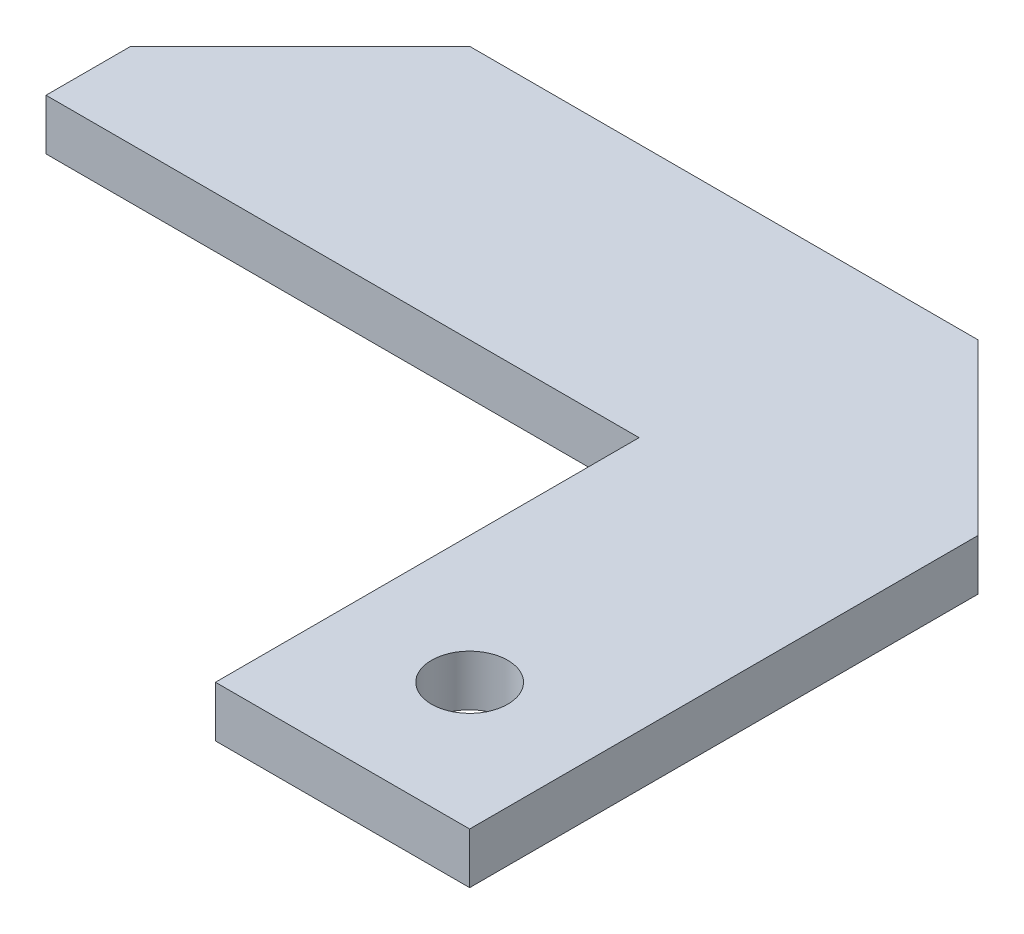
from build123d import *

# Parameters (mm, degrees)
BOSS_EXTRUDE1_DEPTH = 6
SKETCH2_R           = 4.5
CUT_EXTRUDE1_DEPTH  = 6
CHAMFER1_SIZE       = 20
CHAMFER2_SIZE       = 20


with BuildPart() as part:
    # Sketch1 → Boss-Extrude1 (new body)
    with BuildSketch(Plane(origin=(0, 0, 0), x_dir=(1, 0, 0), z_dir=(0, 1, 0))):
        Polygon((-18.076923077, 61.923076923), (81.923076923, 61.923076923), (81.923076923, -18.076923077), (51.923076923, -18.076923077), (51.923076923, 31.923076923), (-18.076923077, 31.923076923), align=None)
    extrude(amount=BOSS_EXTRUDE1_DEPTH)

    # Sketch2 → Cut-Extrude1 (cut)
    with BuildSketch(Plane(origin=(0, 6, 0), x_dir=(1, 0, 0), z_dir=(0, 1, 0))):
        with Locations(Location((66.923076923, -3.076923077, 0), (0, 0, 270))):
            Circle(SKETCH2_R)
    extrude(amount=-CUT_EXTRUDE1_DEPTH, mode=Mode.SUBTRACT)

    # Chamfer1
    chamfer1_edges = [part.edges().sort_by_distance(p)[0] for p in [
        (-18.076923077, 3, -61.923076923),
    ]]
    chamfer(chamfer1_edges, length=CHAMFER1_SIZE)

    # Chamfer2
    chamfer2_edges = [part.edges().sort_by_distance(p)[0] for p in [
        (81.923076923, 3, -61.923076923),
    ]]
    chamfer(chamfer2_edges, length=CHAMFER2_SIZE)


solid = part.part
